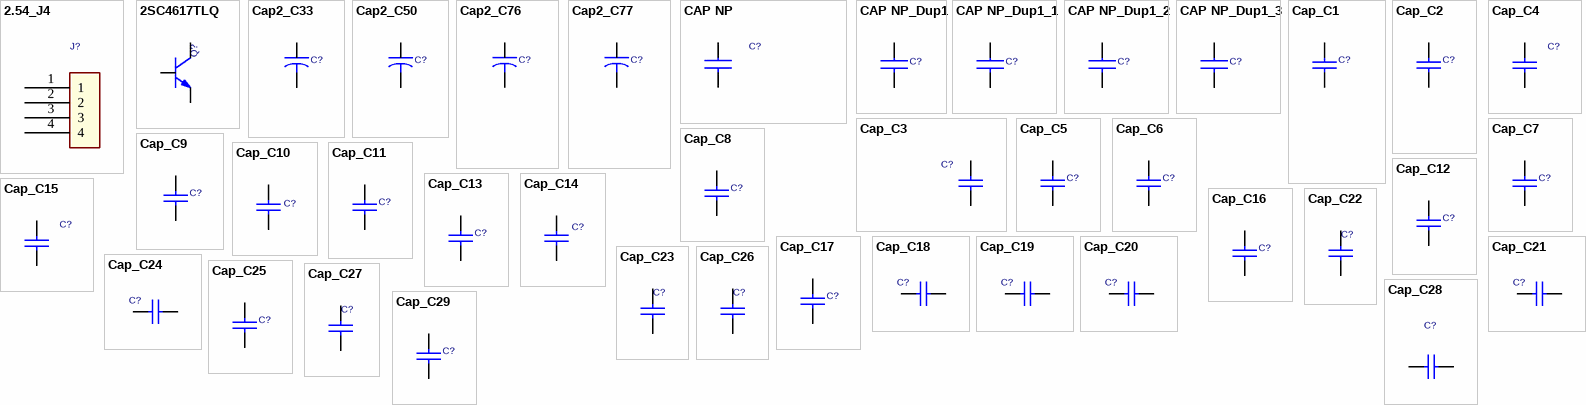
[diagram p0: symbols 2.54_J4 to Cap_C29]
# Altium schematic symbol library MISC86294-22.SCHLIB: 224 symbols
Pins are listed as number, name and electrical type; pins without a type are passive.


## 2.54_J4
designator J?
footprint HDR1X4
pins: 1, 2, 3, 4

## 2SC4617TLQ
designator Q?
simulation model 2SC4617TLQ
footprint EMT3
pins: 1 E, 2 B, 3 C

## Cap2_C33
designator C?
footprint CAP-TH_BD5_0-P2_00-D0_8-FD
pins: 1, 2

## Cap2_C50
designator C?
footprint C0805
pins: 1, 2

## Cap2_C76
designator C?
footprint RB5*7
pins: 1, 2

## Cap2_C77
designator C?
footprint RB5*7
pins: 1, 2

## CAP NP
designator C?
footprint 0603
pins: 1, 2

## CAP NP_Dup1
designator C?
footprint C0603
pins: 1, 2

## CAP NP_Dup1_1
designator C?
footprint C0603
pins: 1, 2

## CAP NP_Dup1_2
designator C?
footprint C0603
pins: 1, 2

## CAP NP_Dup1_3
designator C?
footprint C0805
pins: 1, 2

## Cap_C1
designator C?
footprint C0805
pins: 1, 2

## Cap_C2
designator C?
footprint C0805
pins: 1, 2

## Cap_C3
designator C?
footprint C0805
pins: 1, 2

## Cap_C4
designator C?
footprint C0805
pins: 1, 2

## Cap_C5
designator C?
footprint 0603
footprint C0603
pins: 1, 2

## Cap_C6
designator C?
footprint 0603
footprint C0603
pins: 1, 2

## Cap_C7
designator C?
footprint 0603
footprint C0603
pins: 1, 2

## Cap_C8
designator C?
footprint 0603
footprint C0603
pins: 1, 2

## Cap_C9
designator C?
footprint 0603
footprint C0603
pins: 1, 2

## Cap_C10
designator C?
footprint 0603
footprint C0603
pins: 1, 2

## Cap_C11
designator C?
footprint 0603
footprint C0603
pins: 1, 2

## Cap_C12
designator C?
footprint 0603
footprint C0603
pins: 1, 2

## Cap_C13
designator C?
footprint 0603
footprint C0603
pins: 1, 2

## Cap_C14
designator C?
footprint 0603
footprint C0603
pins: 1, 2

## Cap_C15
designator C?
footprint C0805
pins: 1, 2

## Cap_C16
designator C?
footprint 0603
footprint C0603
pins: 1, 2

## Cap_C17
designator C?
footprint 0603
footprint C0603
pins: 1, 2

## Cap_C18
designator C?
footprint 0603
pins: 1, 2

## Cap_C19
designator C?
footprint 0603
pins: 1, 2

## Cap_C20
designator C?
footprint 0603
pins: 1, 2

## Cap_C21
designator C?
footprint 0603
pins: 1, 2

## Cap_C22
designator C?
footprint 0603
pins: 1, 2

## Cap_C23
designator C?
footprint 0603
pins: 1, 2

## Cap_C24
designator C?
footprint 0603
pins: 1, 2

## Cap_C25
designator C?
footprint CAP-TH_BD8_0-P3_50-D1_0-FD
pins: 1, 2

## Cap_C26
designator C?
footprint 0603
pins: 1, 2

## Cap_C27
designator C?
footprint 0603
pins: 1, 2

## Cap_C28
designator C?
footprint 0603
footprint C0603
pins: 1, 2

## Cap_C29
designator C?
footprint 0603
footprint C0603
pins: 1, 2

## Cap_C30
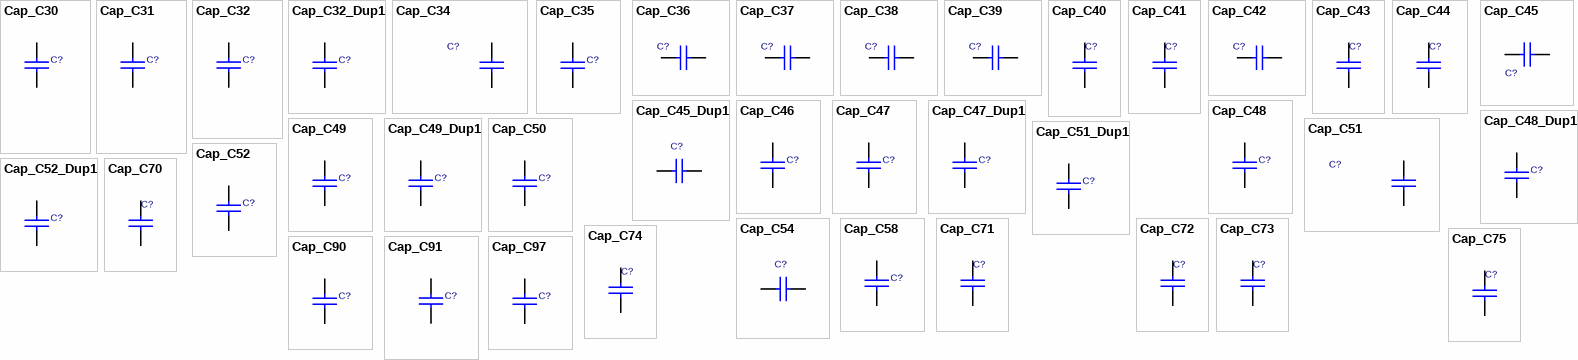
[diagram p1: symbols Cap_C30 to Cap_C97]
## Cap_C30
designator C?
footprint C0805
pins: 1, 2

## Cap_C31
designator C?
footprint 0603
footprint C0603
pins: 1, 2

## Cap_C32
designator C?
footprint C0805
pins: 1, 2

## Cap_C32_Dup1
designator C?
footprint C0603
pins: 1, 2

## Cap_C34
designator C?
footprint C0805
pins: 1, 2

## Cap_C35
designator C?
footprint 0603
footprint C0603
pins: 1, 2

## Cap_C36
designator C?
footprint 0603
pins: 1, 2

## Cap_C37
designator C?
footprint 0603
pins: 1, 2

## Cap_C38
designator C?
footprint 0603
pins: 1, 2

## Cap_C39
designator C?
footprint 0603
pins: 1, 2

## Cap_C40
designator C?
footprint 0603
pins: 1, 2

## Cap_C41
designator C?
footprint 0603
pins: 1, 2

## Cap_C42
designator C?
footprint 0603
pins: 1, 2

## Cap_C43
designator C?
footprint 0603
pins: 1, 2

## Cap_C44
designator C?
footprint 0603
pins: 1, 2

## Cap_C45
designator C?
footprint 0603
footprint C0603
pins: 1, 2

## Cap_C45_Dup1
designator C?
footprint C0603
pins: 1, 2

## Cap_C46
designator C?
footprint 0603
footprint C0603
pins: 1, 2

## Cap_C47
designator C?
footprint C0805
pins: 1, 2

## Cap_C47_Dup1
designator C?
footprint C0603
pins: 1, 2

## Cap_C48
designator C?
footprint 0603
footprint C0603
pins: 1, 2

## Cap_C48_Dup1
designator C?
footprint C0603
pins: 1, 2

## Cap_C49
designator C?
footprint C0805
pins: 1, 2

## Cap_C49_Dup1
designator C?
footprint C0603
pins: 1, 2

## Cap_C50
designator C?
footprint C0603
pins: 1, 2

## Cap_C51
designator C?
footprint C0805
pins: 1, 2

## Cap_C51_Dup1
designator C?
footprint C0603
pins: 1, 2

## Cap_C52
designator C?
footprint 0603
footprint C0603
pins: 1, 2

## Cap_C52_Dup1
designator C?
footprint C0603
pins: 1, 2

## Cap_C54
designator C?
footprint C0603
pins: 1, 2

## Cap_C58
designator C?
footprint C0603
pins: 1, 2

## Cap_C70
designator C?
footprint C0603
pins: 1, 2

## Cap_C71
designator C?
footprint C0603
pins: 1, 2

## Cap_C72
designator C?
footprint C0603
pins: 1, 2

## Cap_C73
designator C?
footprint C0603
pins: 1, 2

## Cap_C74
designator C?
footprint C0603
pins: 1, 2

## Cap_C75
designator C?
footprint C0603
pins: 1, 2

## Cap_C90
designator C?
footprint C0603
pins: 1, 2

## Cap_C91
designator C?
footprint RB8*11_5
pins: 1, 2

## Cap_C97
designator C?
footprint C0603
pins: 1, 2

## Cap_C98
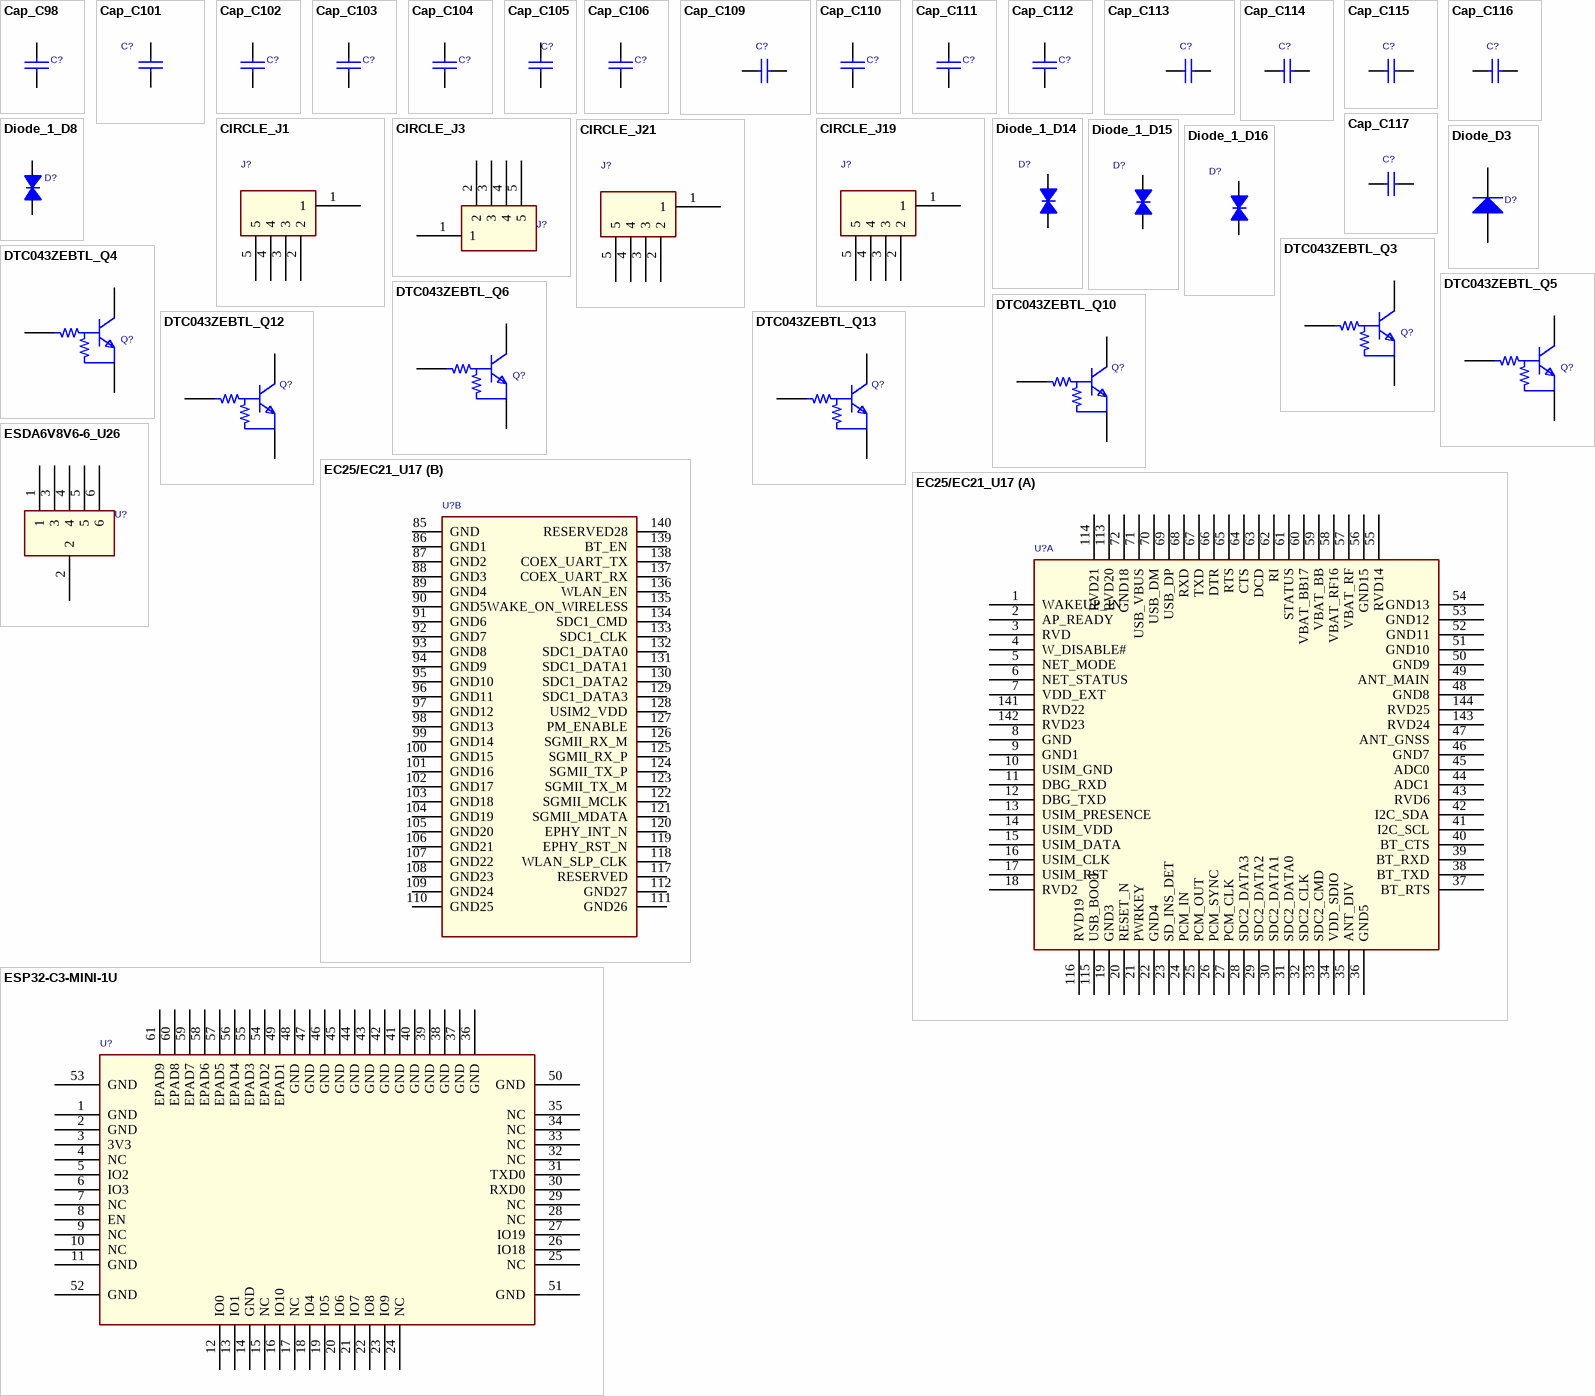
[diagram p2: symbols Cap_C98 to ESP32-C3-MINI-1U]
## Cap_C98
designator C?
footprint C0603
pins: 1, 2

## Cap_C101
designator C?
footprint C0603
pins: 1, 2

## Cap_C102
designator C?
footprint C0603
pins: 1, 2

## Cap_C103
designator C?
footprint C0603
pins: 1, 2

## Cap_C104
designator C?
footprint RB8*11_5
pins: 1, 2

## Cap_C105
designator C?
footprint C0603
pins: 1, 2

## Cap_C106
designator C?
footprint C0603
pins: 1, 2

## Cap_C109
designator C?
footprint C0603
pins: 1, 2

## Cap_C110
designator C?
footprint C0603
pins: 1, 2

## Cap_C111
designator C?
footprint C0603
pins: 1, 2

## Cap_C112
designator C?
footprint C0603
pins: 1, 2

## Cap_C113
designator C?
footprint C0603
pins: 1, 2

## Cap_C114
designator C?
footprint C0603
pins: 1, 2

## Cap_C115
designator C?
footprint C0603
pins: 1, 2

## Cap_C116
designator C?
footprint C0603
pins: 1, 2

## Cap_C117
designator C?
footprint C0603
pins: 1, 2

## CIRCLE_J1
designator J?
footprint MMCX-TH_ZC11_801KK
pins: 1, 2, 3, 4, 5

## CIRCLE_J3
designator J?
footprint MMCX-TH_ZC11_801KK
pins: 1, 2, 3, 4, 5

## CIRCLE_J19
designator J?
footprint MMCX-KE
pins: 1, 2, 3, 4, 5

## CIRCLE_J21
designator J?
footprint MMCX-KE
pins: 1, 2, 3, 4, 5

## Diode_1_D8
designator D?
footprint SMA
pins: 1 A, 2 K

## Diode_1_D14
designator D?
footprint SMA
pins: 1 A, 2 K

## Diode_1_D15
designator D?
footprint SMA
pins: 1 A, 2 K

## Diode_1_D16
designator D?
footprint SMA
pins: 1 A, 2 K

## Diode_D3
designator D?
footprint SMC_L6_9-W5_9-LS7_9-RD
pins: 1 A, 2 K

## DTC043ZEBTL_Q3
designator Q?
footprint SOT-416_L1_6-W0_8-P1_00-LS1_6-BR
pins: 1 B, 2 E, 3 C

## DTC043ZEBTL_Q4
designator Q?
footprint SOT-416_L1_6-W0_8-P1_00-LS1_6-BR
pins: 1 B, 2 E, 3 C

## DTC043ZEBTL_Q5
designator Q?
footprint SOT-416_L1_6-W0_8-P1_00-LS1_6-BR
pins: 1 B, 2 E, 3 C

## DTC043ZEBTL_Q6
designator Q?
footprint SOT-416_L1_6-W0_8-P1_00-LS1_6-BR
pins: 1 B, 2 E, 3 C

## DTC043ZEBTL_Q10
designator Q?
footprint SOT-416_L1_6-W0_8-P1_00-LS1_6-BR
pins: 1 B, 2 E, 3 C

## DTC043ZEBTL_Q12
designator Q?
footprint SOT-416_L1_6-W0_8-P1_00-LS1_6-BR
pins: 1 B, 2 E, 3 C

## DTC043ZEBTL_Q13
designator Q?
footprint SOT-416_L1_6-W0_8-P1_00-LS1_6-BR
pins: 1 B, 2 E, 3 C

## EC25/EC21_U17
designator U?
footprint EC20
part A pins: 1 WAKEUP_IN, 2 AP_READY, 3 RVD, 4 W_DISABLE#, 5 NET_MODE, 6 NET_STATUS, 7 VDD_EXT, 8 GND, 9 GND1, 10 USIM_GND, 11 DBG_RXD, 12 DBG_TXD, 13 USIM_PRESENCE, 14 USIM_VDD, 15 USIM_DATA, 16 USIM_CLK, 17 USIM_RST, 18 RVD2, 19 GND3, 20 RESET_N, 21 PWRKEY, 22 GND4, 23 SD_INS_DET, 24 PCM_IN, 25 PCM_OUT, 26 PCM_SYNC, 27 PCM_CLK, 28 SDC2_DATA3, 29 SDC2_DATA2, 30 SDC2_DATA1, 31 SDC2_DATA0, 32 SDC2_CLK, 33 SDC2_CMD, 34 VDD_SDIO, 35 ANT_DIV, 36 GND5, 37 BT_RTS, 38 BT_TXD, 39 BT_RXD, 40 BT_CTS, 41 I2C_SCL, 42 I2C_SDA, 43 RVD6, 44 ADC1, 45 ADC0, 46 GND7, 47 ANT_GNSS, 48 GND8, 49 ANT_MAIN, 50 GND9, 51 GND10, 52 GND11, 53 GND12, 54 GND13, 55 RVD14, 56 GND15, 57 VBAT_RF, 58 VBAT_RF16, 59 VBAT_BB, 60 VBAT_BB17, 61 STATUS, 62 RI, 63 DCD, 64 CTS, 65 RTS, 66 DTR, 67 TXD, 68 RXD, 69 USB_DP, 70 USB_DM, 71 USB_VBUS, 72 GND18, 113 RVD20, 114 RVD21, 115 USB_BOOT, 116 RVD19, 141 RVD22, 142 RVD23, 143 RVD24, 144 RVD25
part B pins: 85 GND, 86 GND1, 87 GND2, 88 GND3, 89 GND4, 90 GND5, 91 GND6, 92 GND7, 93 GND8, 94 GND9, 95 GND10, 96 GND11, 97 GND12, 98 GND13, 99 GND14, 100 GND15, 101 GND16, 102 GND17, 103 GND18, 104 GND19, 105 GND20, 106 GND21, 107 GND22, 108 GND23, 109 GND24, 110 GND25, 111 GND26, 112 GND27, 117 RESERVED, 118 WLAN_SLP_CLK, 119 EPHY_RST_N, 120 EPHY_INT_N, 121 SGMII_MDATA, 122 SGMII_MCLK, 123 SGMII_TX_M, 124 SGMII_TX_P, 125 SGMII_RX_P, 126 SGMII_RX_M, 127 PM_ENABLE, 128 USIM2_VDD, 129 SDC1_DATA3, 130 SDC1_DATA2, 131 SDC1_DATA1, 132 SDC1_DATA0, 133 SDC1_CLK, 134 SDC1_CMD, 135 WAKE_ON_WIRELESS, 136 WLAN_EN, 137 COEX_UART_RX, 138 COEX_UART_TX, 139 BT_EN, 140 RESERVED28

## ESDA6V8V6-6_U26
designator U?
footprint SOT-563
pins: 1, 2, 3, 4, 5, 6

## ESP32-C3-MINI-1U
designator U?
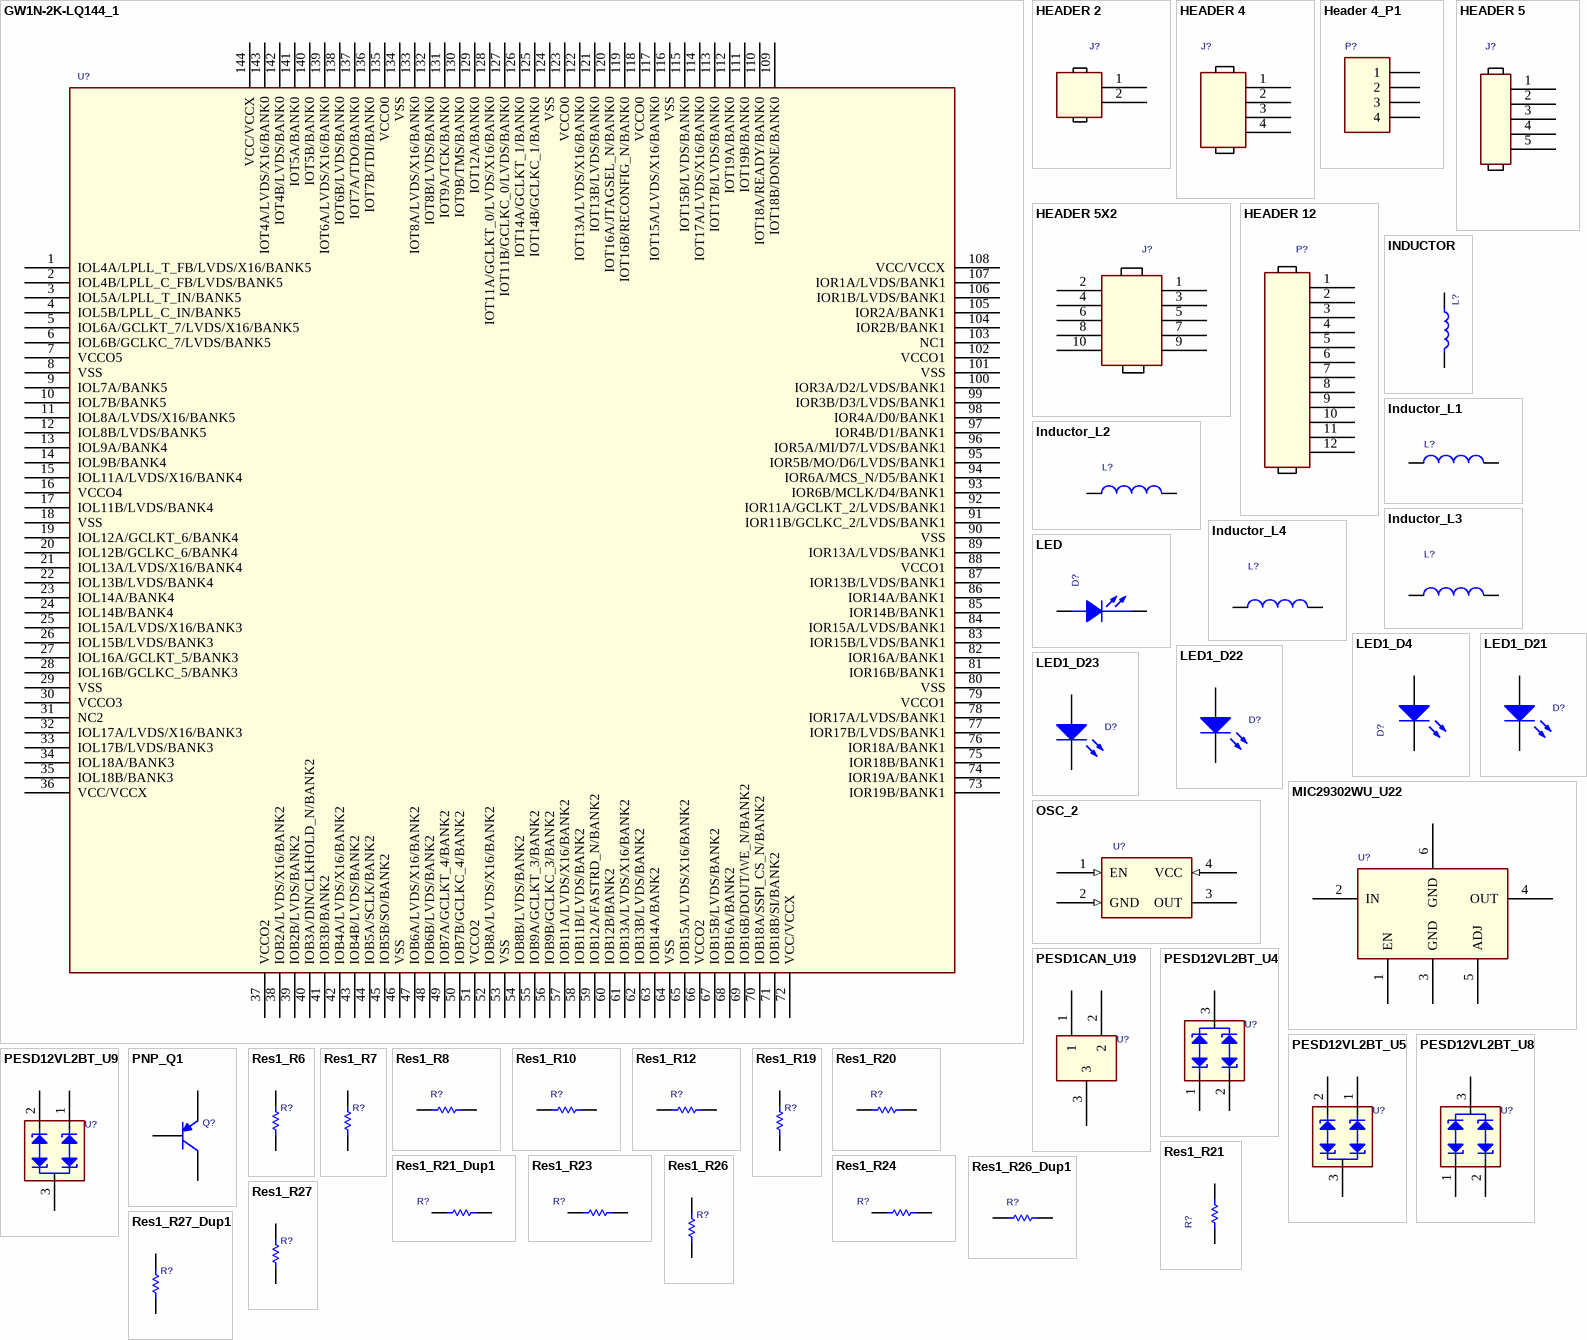
[diagram p3: symbols GW1N-2K-LQ144_1 to Res1_R27_Dup1]
pins: 1 GND, 2 GND, 3 3V3, 4 NC, 5 IO2, 6 IO3, 7 NC, 8 EN, 9 NC, 10 NC, 11 GND, 12 IO0, 13 IO1, 14 GND, 15 NC, 16 IO10, 17 NC, 18 IO4, 19 IO5, 20 IO6, 21 IO7, 22 IO8, 23 IO9, 24 NC, 25 NC, 26 IO18, 27 IO19, 28 NC, 29 NC, 30 RXD0, 31 TXD0, 32 NC, 33 NC, 34 NC, 35 NC, 36 GND, 37 GND, 38 GND, 39 GND, 40 GND, 41 GND, 42 GND, 43 GND, 44 GND, 45 GND, 46 GND, 47 GND, 48 GND, 49 EPAD1, 50 GND, 51 GND, 52 GND, 53 GND, 54 EPAD2, 55 EPAD3, 56 EPAD4, 57 EPAD5, 58 EPAD6, 59 EPAD7, 60 EPAD8, 61 EPAD9


## GW1N-2K-LQ144_1
designator U?
footprint LQ144_1
pins: 1 IOL4A/LPLL_T_FB/LVDS/X16/BANK5, 2 IOL4B/LPLL_C_FB/LVDS/BANK5, 3 IOL5A/LPLL_T_IN/BANK5, 4 IOL5B/LPLL_C_IN/BANK5, 5 IOL6A/GCLKT_7/LVDS/X16/BANK5, 6 IOL6B/GCLKC_7/LVDS/BANK5, 7 VCCO5 (power), 8 VSS (power), 9 IOL7A/BANK5, 10 IOL7B/BANK5, 11 IOL8A/LVDS/X16/BANK5, 12 IOL8B/LVDS/BANK5, 13 IOL9A/BANK4, 14 IOL9B/BANK4, 15 IOL11A/LVDS/X16/BANK4, 16 VCCO4 (power), 17 IOL11B/LVDS/BANK4, 18 VSS (power), 19 IOL12A/GCLKT_6/BANK4, 20 IOL12B/GCLKC_6/BANK4, 21 IOL13A/LVDS/X16/BANK4, 22 IOL13B/LVDS/BANK4, 23 IOL14A/BANK4, 24 IOL14B/BANK4, 25 IOL15A/LVDS/X16/BANK3, 26 IOL15B/LVDS/BANK3, 27 IOL16A/GCLKT_5/BANK3, 28 IOL16B/GCLKC_5/BANK3, 29 VSS (power), 30 VCCO3 (power), 31 NC2, 32 IOL17A/LVDS/X16/BANK3, 33 IOL17B/LVDS/BANK3, 34 IOL18A/BANK3, 35 IOL18B/BANK3, 36 VCC/VCCX (power), 37 VCCO2 (power), 38 IOB2A/LVDS/X16/BANK2, 39 IOB2B/LVDS/BANK2, 40 IOB3A/DIN/CLKHOLD_N/BANK2, 41 IOB3B/BANK2, 42 IOB4A/LVDS/X16/BANK2, 43 IOB4B/LVDS/BANK2, 44 IOB5A/SCLK/BANK2, 45 IOB5B/SO/BANK2, 46 VSS (power), 47 IOB6A/LVDS/X16/BANK2, 48 IOB6B/LVDS/BANK2, 49 IOB7A/GCLKT_4/BANK2, 50 IOB7B/GCLKC_4/BANK2, 51 VCCO2 (power), 52 IOB8A/LVDS/X16/BANK2, 53 VSS (power), 54 IOB8B/LVDS/BANK2, 55 IOB9A/GCLKT_3/BANK2, 56 IOB9B/GCLKC_3/BANK2, 57 IOB11A/LVDS/X16/BANK2, 58 IOB11B/LVDS/BANK2, 59 IOB12A/FASTRD_N/BANK2, 60 IOB12B/BANK2, 61 IOB13A/LVDS/X16/BANK2, 62 IOB13B/LVDS/BANK2, 63 IOB14A/BANK2, 64 VSS (power), 65 IOB15A/LVDS/X16/BANK2, 66 VCCO2 (power), 67 IOB15B/LVDS/BANK2, 68 IOB16A/BANK2, 69 IOB16B/DOUT/WE_N/BANK2, 70 IOB18A/SSPI_CS_N/BANK2, 71 IOB18B/SI/BANK2, 72 VCC/VCCX (power), 73 IOR19B/BANK1, 74 IOR19A/BANK1, 75 IOR18B/BANK1, 76 IOR18A/BANK1, 77 IOR17B/LVDS/BANK1, 78 IOR17A/LVDS/BANK1, 79 VCCO1 (power), 80 VSS (power), 81 IOR16B/BANK1, 82 IOR16A/BANK1, 83 IOR15B/LVDS/BANK1, 84 IOR15A/LVDS/BANK1, 85 IOR14B/BANK1, 86 IOR14A/BANK1, 87 IOR13B/LVDS/BANK1, 88 VCCO1 (power), 89 IOR13A/LVDS/BANK1, 90 VSS (power), 91 IOR11B/GCLKC_2/LVDS/BANK1, 92 IOR11A/GCLKT_2/LVDS/BANK1, 93 IOR6B/MCLK/D4/BANK1, 94 IOR6A/MCS_N/D5/BANK1, 95 IOR5B/MO/D6/LVDS/BANK1, 96 IOR5A/MI/D7/LVDS/BANK1, 97 IOR4B/D1/BANK1, 98 IOR4A/D0/BANK1, 99 IOR3B/D3/LVDS/BANK1, 100 IOR3A/D2/LVDS/BANK1, 101 VSS (power), 102 VCCO1 (power), 103 NC1, 104 IOR2B/BANK1, 105 IOR2A/BANK1, 106 IOR1B/LVDS/BANK1, 107 IOR1A/LVDS/BANK1, 108 VCC/VCCX (power), 109 IOT18B/DONE/BANK0, 110 IOT18A/READY/BANK0, 111 IOT19B/BANK0, 112 IOT19A/BANK0, 113 IOT17B/LVDS/BANK0, 114 IOT17A/LVDS/X16/BANK0, 115 IOT15B/LVDS/BANK0, 116 VSS (power), 117 IOT15A/LVDS/X16/BANK0, 118 VCCO0 (power), 119 IOT16B/RECONFIG_N/BANK0, 120 IOT16A/JTAGSEL_N/BANK0, 121 IOT13B/LVDS/BANK0, 122 IOT13A/LVDS/X16/BANK0, 123 VCCO0 (power), 124 VSS (power), 125 IOT14B/GCLKC_1/BANK0, 126 IOT14A/GCLKT_1/BANK0, 127 IOT11B/GCLKC_0/LVDS/BANK0, 128 IOT11A/GCLKT_0/LVDS/X16/BANK0, 129 IOT12A/BANK0, 130 IOT9B/TMS/BANK0, 131 IOT9A/TCK/BANK0, 132 IOT8B/LVDS/BANK0, 133 IOT8A/LVDS/X16/BANK0, 134 VSS (power), 135 VCCO0 (power), 136 IOT7B/TDI/BANK0, 137 IOT7A/TDO/BANK0, 138 IOT6B/LVDS/BANK0, 139 IOT6A/LVDS/X16/BANK0, 140 IOT5B/BANK0, 141 IOT5A/BANK0, 142 IOT4B/LVDS/BANK0, 143 IOT4A/LVDS/X16/BANK0, 144 VCC/VCCX (power)

## HEADER 2
designator J?
pins: 1, 2

## HEADER 4
designator J?
pins: 1, 2, 3, 4

## Header 4_P1
designator P?
footprint HDR1X4
pins: 1, 2, 3, 4

## HEADER 5
designator J?
footprint 2.54mm_paizhen_5pin
pins: 1, 2, 3, 4, 5

## HEADER 5X2
designator J?
pins: 1, 2, 3, 4, 5, 6, 7, 8, 9, 10

## HEADER 12
designator P?
pins: 1, 2, 3, 4, 5, 6, 7, 8, 9, 10, 11, 12

## INDUCTOR
designator L?
footprint 0805
pins: 1, 2

## Inductor_L1
designator L?
footprint 1210
pins: 1, 2

## Inductor_L2
designator L?
footprint 0603
footprint R0603
pins: 1, 2

## Inductor_L3
designator L?
footprint IND-SMD_L4_0-W4_0
pins: 1, 2

## Inductor_L4
designator L?
footprint IND-SMD_L4_0-W4_0
pins: 1, 2

## LED
designator D?
footprint LED0603
pins: 1 CATHODE, 2 ANODE

## LED1_D4
designator D?
footprint LED_0805
footprint LED0603
pins: 1 A, 2 K

## LED1_D21
designator D?
footprint LED0805
pins: 1 A, 2 K

## LED1_D22
designator D?
footprint LED0805
pins: 1 A, 2 K

## LED1_D23
designator D?
footprint LED0805
pins: 1 A, 2 K

## MIC29302WU_U22
designator U?
footprint TO-263-5
pins: 1 EN, 2 IN, 3 GND, 4 OUT, 5 ADJ, 6 GND

## OSC_2
designator U?
100Mhz Oscillator half can
footprint SMD3225
pins: 1 EN (in), 2 GND (in), 3 OUT, 4 VCC (in)

## PESD1CAN_U19
designator U?
footprint SOT-23-3
pins: 1, 2, 3

## PESD12VL2BT_U4
designator U?
footprint SOT-23
pins: 1, 2, 3

## PESD12VL2BT_U5
designator U?
footprint SOT-23
pins: 1, 2, 3

## PESD12VL2BT_U8
designator U?
footprint SOT-23
pins: 1, 2, 3

## PESD12VL2BT_U9
designator U?
footprint SOT-23
pins: 1, 2, 3

## PNP_Q1
designator Q?
footprint SOT-23-SS8550
pins: 1 B, 2 E, 3 C

## Res1_R6
designator R?
footprint 0603
pins: 1, 2

## Res1_R7
designator R?
footprint 0603
pins: 1, 2

## Res1_R8
designator R?
footprint 0603
pins: 1, 2

## Res1_R10
designator R?
footprint 0603
pins: 1, 2

## Res1_R12
designator R?
footprint 0603
pins: 1, 2

## Res1_R19
designator R?
footprint 0603
footprint R0603
pins: 1, 2

## Res1_R20
designator R?
footprint 0603
footprint R0603
pins: 1, 2

## Res1_R21
designator R?
footprint 0603
pins: 1, 2

## Res1_R21_Dup1
designator R?
footprint R0603
pins: 1, 2

## Res1_R23
designator R?
footprint R0603
pins: 1, 2

## Res1_R24
designator R?
footprint R0603
pins: 1, 2

## Res1_R26
designator R?
footprint 0603
footprint R0603
pins: 1, 2

## Res1_R26_Dup1
designator R?
footprint R0603
pins: 1, 2

## Res1_R27
designator R?
footprint 0603
footprint R0603
pins: 1, 2

## Res1_R27_Dup1
designator R?
footprint R0603
pins: 1, 2

## Res1_R28
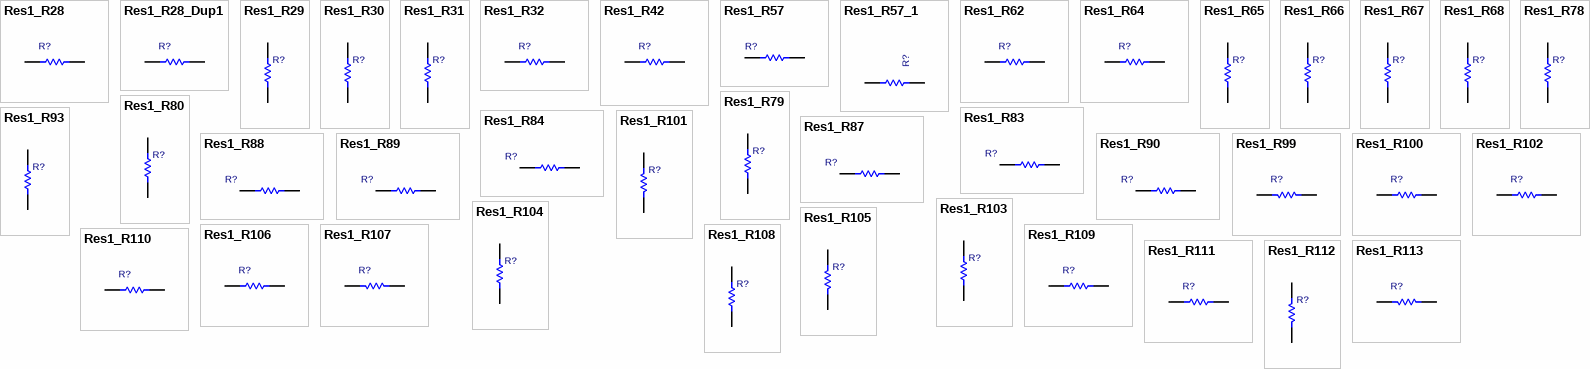
[diagram p4: symbols Res1_R28 to Res1_R113]
## Res1_R28
designator R?
footprint 0603
footprint R0603
pins: 1, 2

## Res1_R28_Dup1
designator R?
footprint R0603
pins: 1, 2

## Res1_R29
designator R?
footprint 0603
footprint R0603
pins: 1, 2

## Res1_R30
designator R?
footprint R0603
pins: 1, 2

## Res1_R31
designator R?
footprint R0603
pins: 1, 2

## Res1_R32
designator R?
footprint R0603
pins: 1, 2

## Res1_R42
designator R?
footprint R0603
pins: 1, 2

## Res1_R57
designator R?
footprint R0603
pins: 1, 2

## Res1_R57_1
designator R?
footprint R0603
pins: 1, 2

## Res1_R62
designator R?
footprint R0603
pins: 1, 2

## Res1_R64
designator R?
footprint R0603
pins: 1, 2

## Res1_R65
designator R?
footprint R0603
pins: 1, 2

## Res1_R66
designator R?
footprint R0603
pins: 1, 2

## Res1_R67
designator R?
footprint R0603
pins: 1, 2

## Res1_R68
designator R?
footprint R0603
pins: 1, 2

## Res1_R78
designator R?
footprint R0603
pins: 1, 2

## Res1_R79
designator R?
footprint R0603
pins: 1, 2

## Res1_R80
designator R?
footprint R0603
pins: 1, 2

## Res1_R83
designator R?
footprint R0603
pins: 1, 2

## Res1_R84
designator R?
footprint R0603
pins: 1, 2

## Res1_R87
designator R?
footprint R0603
pins: 1, 2

## Res1_R88
designator R?
footprint R0603
pins: 1, 2

## Res1_R89
designator R?
footprint R0603
pins: 1, 2

## Res1_R90
designator R?
footprint R0603
pins: 1, 2

## Res1_R93
designator R?
footprint R0603
pins: 1, 2

## Res1_R99
designator R?
footprint R0603
pins: 1, 2

## Res1_R100
designator R?
footprint R0603
pins: 1, 2

## Res1_R101
designator R?
footprint R0603
pins: 1, 2

## Res1_R102
designator R?
footprint R0603
pins: 1, 2

## Res1_R103
designator R?
footprint R0603
pins: 1, 2

## Res1_R104
designator R?
footprint R0603
pins: 1, 2

## Res1_R105
designator R?
footprint R0603
pins: 1, 2

## Res1_R106
designator R?
footprint R0603
pins: 1, 2

## Res1_R107
designator R?
footprint R0603
pins: 1, 2

## Res1_R108
designator R?
footprint R0603
pins: 1, 2

## Res1_R109
designator R?
footprint R0603
pins: 1, 2

## Res1_R110
designator R?
footprint R0603
pins: 1, 2

## Res1_R111
designator R?
footprint R0603
pins: 1, 2

## Res1_R112
designator R?
footprint R0603
pins: 1, 2

## Res1_R113
designator R?
footprint R0603
pins: 1, 2

## Res1_R114
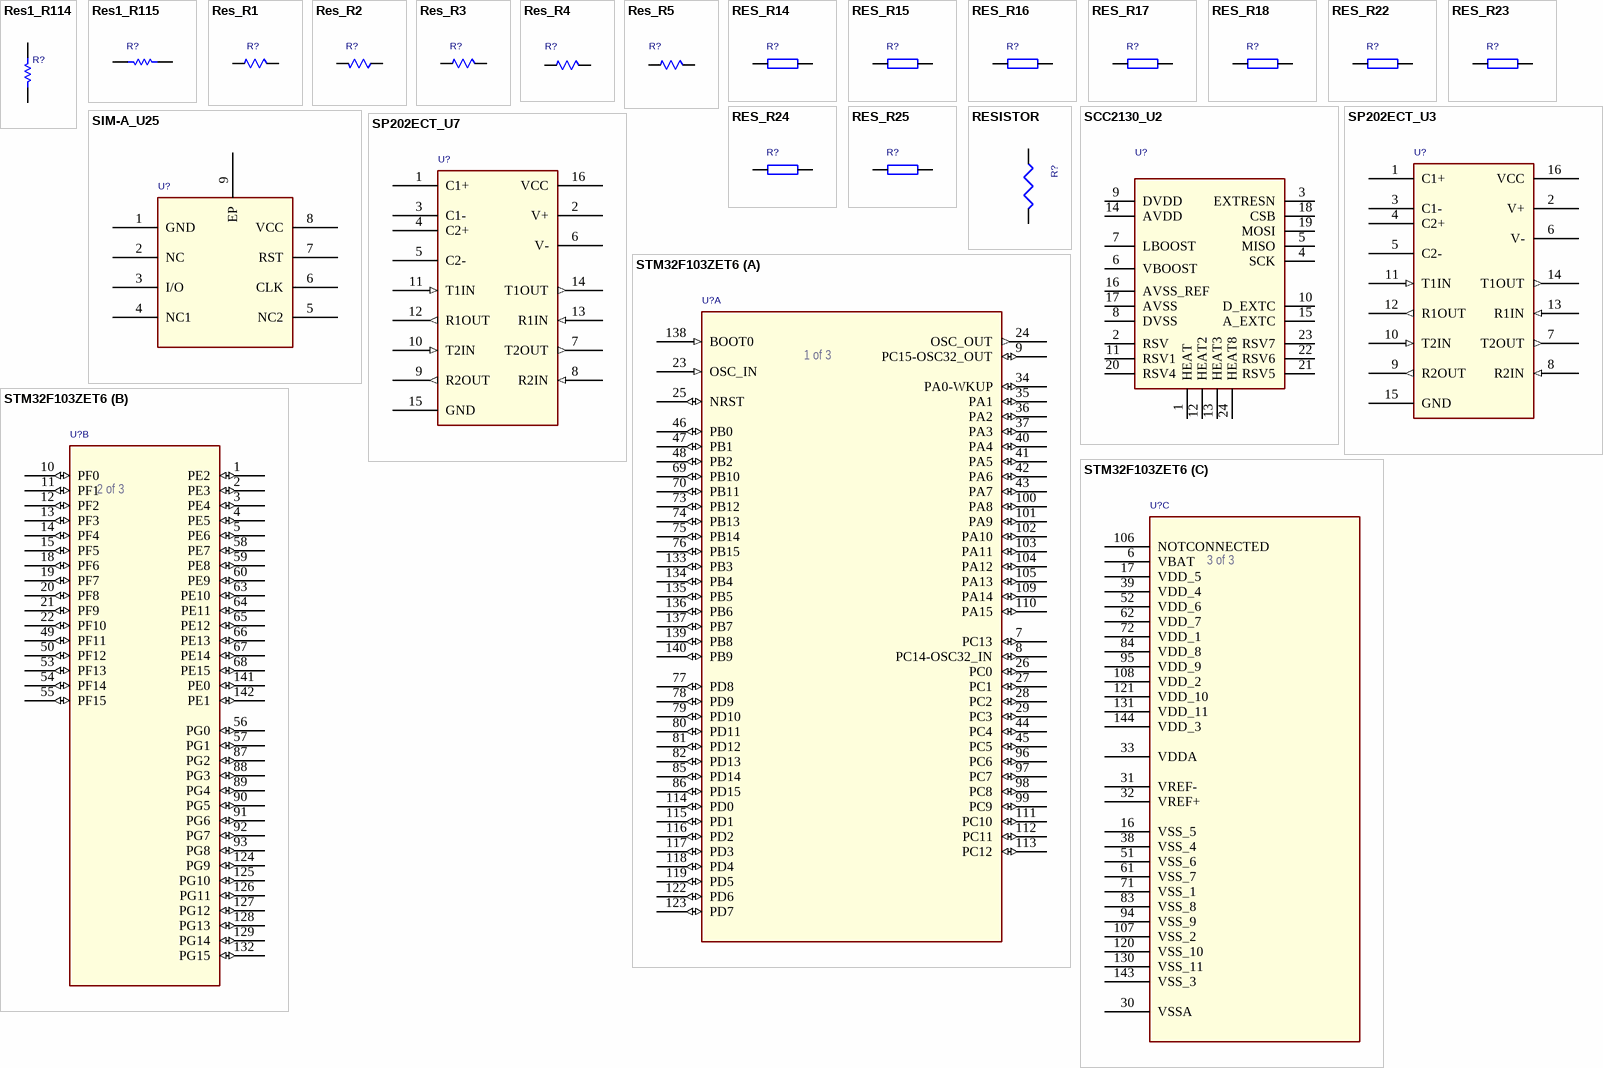
[diagram p5: symbols Res1_R114 to STM32F103ZET6]
## Res1_R114
designator R?
footprint R0603
pins: 1, 2

## Res1_R115
designator R?
footprint R0603
pins: 1, 2

## Res_R1
designator R?
footprint 0603
pins: 1, 2

## Res_R2
designator R?
footprint 0603
pins: 1, 2

## Res_R3
designator R?
footprint 0603
pins: 1, 2

## Res_R4
designator R?
footprint 0603
pins: 1, 2

## Res_R5
designator R?
footprint 0603
pins: 1, 2

## RES_R14
designator R?
footprint 0603
pins: 1, 2

## RES_R15
designator R?
footprint 1210
footprint R1210
pins: 1, 2

## RES_R16
designator R?
footprint 0603
pins: 1, 2

## RES_R17
designator R?
footprint 0603
pins: 1, 2

## RES_R18
designator R?
footprint 0603
pins: 1, 2

## RES_R22
designator R?
footprint 0603
pins: 1, 2

## RES_R23
designator R?
footprint 0603
pins: 1, 2

## RES_R24
designator R?
footprint 0603
pins: 1, 2

## RES_R25
designator R?
footprint 0603
pins: 1, 2

## RESISTOR
designator R?
footprint 0603
pins: 1, 2

## SCC2130_U2
designator U?
footprint SCC2130D
pins: 1 HEAT, 2 RSV, 3 EXTRESN, 4 SCK, 5 MISO, 6 VBOOST, 7 LBOOST, 8 DVSS, 9 DVDD, 10 D_EXTC, 11 RSV1, 12 HEAT2, 13 HEAT3, 14 AVDD, 15 A_EXTC, 16 AVSS_REF, 17 AVSS, 18 CSB, 19 MOSI, 20 RSV4, 21 RSV5, 22 RSV6, 23 RSV7, 24 HEAT8

## SIM-A_U25
designator U?
footprint DFN2*2-8
pins: 1 GND, 2 NC, 3 I/O, 4 NC1, 5 NC2, 6 CLK, 7 RST, 8 VCC, 9 EP

## SP202ECT_U3
designator U?
footprint SOP16-6_6
pins: 1 C1+, 2 V+, 3 C1-, 4 C2+, 5 C2-, 6 V-, 7 T2OUT (out), 8 R2IN (in), 9 R2OUT (out), 10 T2IN (in), 11 T1IN (in), 12 R1OUT (out), 13 R1IN (in), 14 T1OUT (out), 15 GND, 16 VCC

## SP202ECT_U7
designator U?
footprint SOP16-6_6
pins: 1 C1+, 2 V+, 3 C1-, 4 C2+, 5 C2-, 6 V-, 7 T2OUT (out), 8 R2IN (in), 9 R2OUT (out), 10 T2IN (in), 11 T1IN (in), 12 R1OUT (out), 13 R1IN (in), 14 T1OUT (out), 15 GND, 16 VCC

## STM32F103ZET6
designator U?
footprint LQFP144-20x20mm
part A pins: 7 PC13 (io), 8 PC14-OSC32_IN (io), 9 PC15-OSC32_OUT (io), 23 OSC_IN (in), 24 OSC_OUT (out), 25 NRST (io), 26 PC0 (io), 27 PC1 (io), 28 PC2 (io), 29 PC3 (io), 34 PA0-WKUP (io), 35 PA1 (io), 36 PA2 (io), 37 PA3 (io), 40 PA4 (io), 41 PA5 (io), 42 PA6 (io), 43 PA7 (io), 44 PC4 (io), 45 PC5 (io), 46 PB0 (io), 47 PB1 (io), 48 PB2 (io), 69 PB10 (io), 70 PB11 (io), 73 PB12 (io), 74 PB13 (io), 75 PB14 (io), 76 PB15 (io), 77 PD8 (io), 78 PD9 (io), 79 PD10 (io), 80 PD11 (io), 81 PD12 (io), 82 PD13 (io), 85 PD14 (io), 86 PD15 (io), 96 PC6 (io), 97 PC7 (io), 98 PC8 (io), 99 PC9 (io), 100 PA8 (io), 101 PA9 (io), 102 PA10 (io), 103 PA11 (io), 104 PA12 (io), 105 PA13 (io), 109 PA14 (io), 110 PA15 (io), 111 PC10 (io), 112 PC11 (io), 113 PC12 (io), 114 PD0 (io), 115 PD1 (io), 116 PD2 (io), 117 PD3 (io), 118 PD4 (io), 119 PD5 (io), 122 PD6 (io), 123 PD7 (io), 133 PB3 (io), 134 PB4 (io), 135 PB5 (io), 136 PB6 (io), 137 PB7 (io), 138 BOOT0 (in), 139 PB8 (io), 140 PB9 (io)
part B pins: 1 PE2 (io), 2 PE3 (io), 3 PE4 (io), 4 PE5 (io), 5 PE6 (io), 10 PF0 (io), 11 PF1 (io), 12 PF2 (io), 13 PF3 (io), 14 PF4 (io), 15 PF5 (io), 18 PF6 (io), 19 PF7 (io), 20 PF8 (io), 21 PF9 (io), 22 PF10 (io), 49 PF11 (io), 50 PF12 (io), 53 PF13 (io), 54 PF14 (io), 55 PF15 (io), 56 PG0 (io), 57 PG1 (io), 58 PE7 (io), 59 PE8 (io), 60 PE9 (io), 63 PE10 (io), 64 PE11 (io), 65 PE12 (io), 66 PE13 (io), 67 PE14 (io), 68 PE15 (io), 87 PG2 (io), 88 PG3 (io), 89 PG4 (io), 90 PG5 (io), 91 PG6 (io), 92 PG7 (io), 93 PG8 (io), 124 PG9 (io), 125 PG10 (io), 126 PG11 (io), 127 PG12 (io), 128 PG13 (io), 129 PG14 (io), 132 PG15 (io), 141 PE0 (io), 142 PE1 (io)
part C pins: 6 VBAT (power), 16 VSS_5 (power), 17 VDD_5 (power), 30 VSSA (power), 31 VREF- (power), 32 VREF+ (power), 33 VDDA (power), 38 VSS_4 (power), 39 VDD_4 (power), 51 VSS_6 (power), 52 VDD_6 (power), 61 VSS_7 (power), 62 VDD_7 (power), 71 VSS_1 (power), 72 VDD_1 (power), 83 VSS_8 (power), 84 VDD_8 (power), 94 VSS_9 (power), 95 VDD_9 (power), 106 NOTCONNECTED, 107 VSS_2 (power), 108 VDD_2 (power), 120 VSS_10 (power), 121 VDD_10 (power), 130 VSS_11 (power), 131 VDD_11 (power), 143 VSS_3 (power), 144 VDD_3 (power)

## STM32F407ZET6
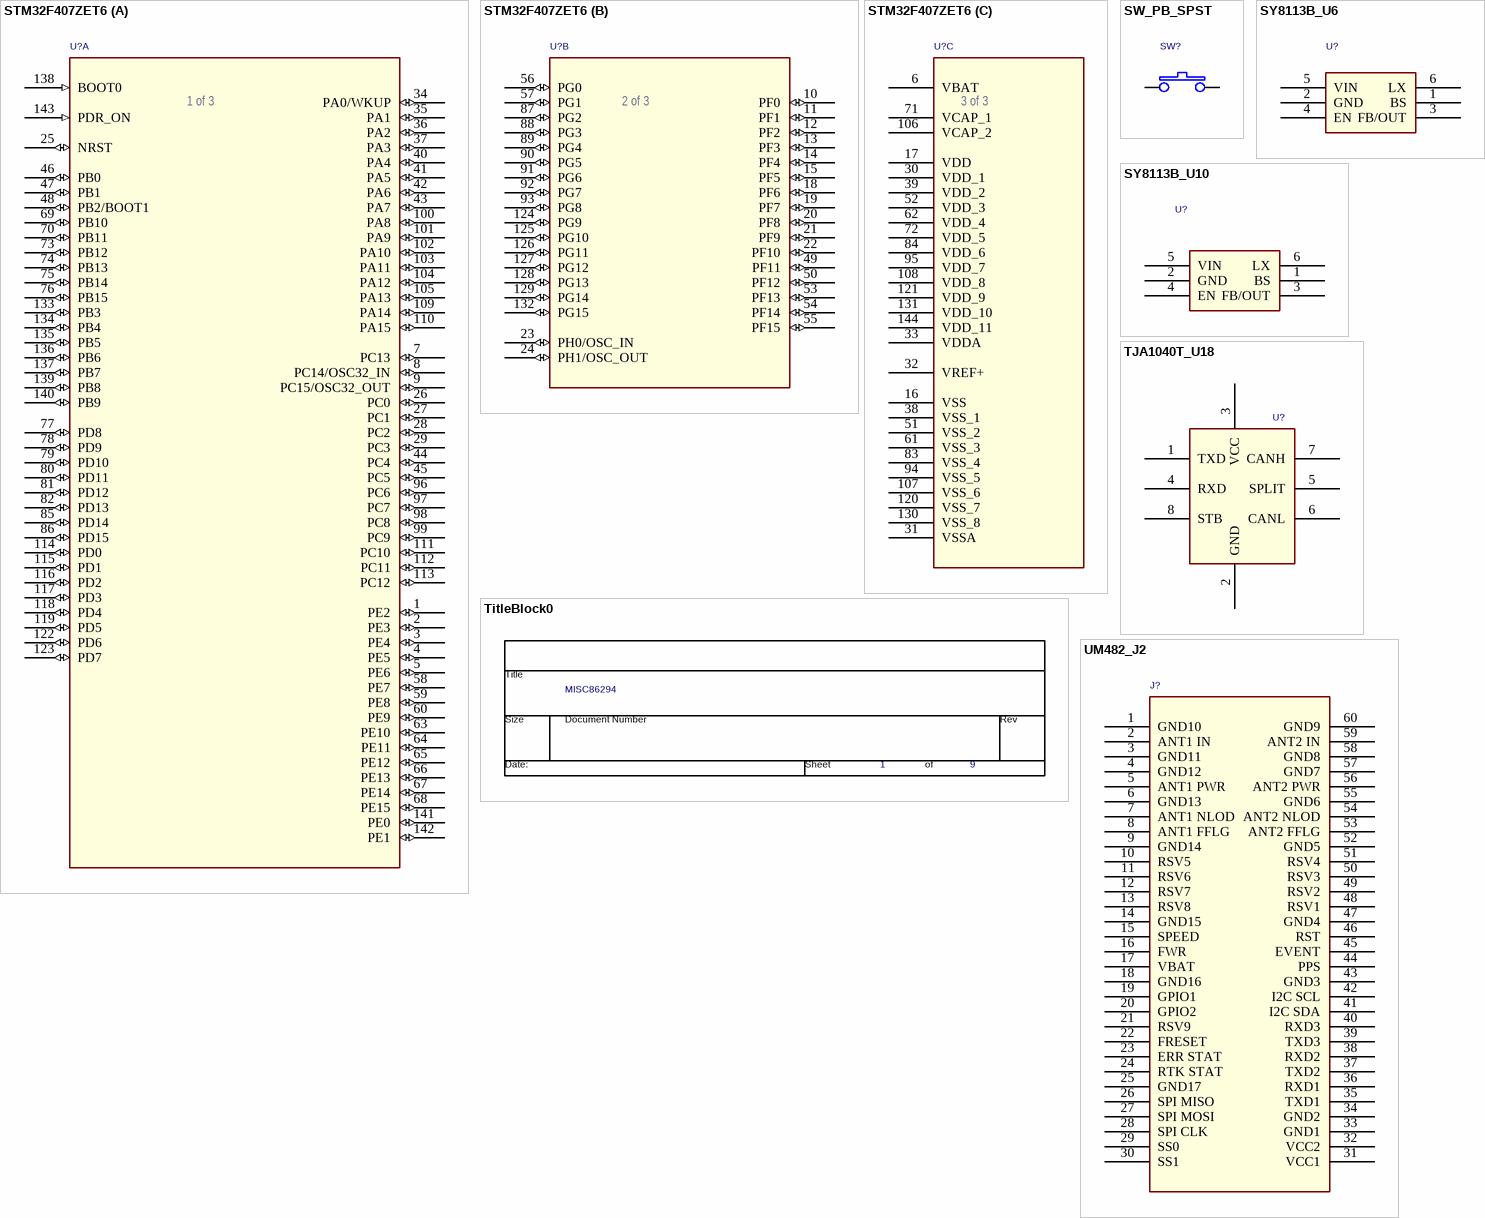
[diagram p6: symbols STM32F407ZET6 to UM482_J2]
## STM32F407ZET6
designator U?
footprint LQFP144-20x20mm
part A pins: 1 PE2 (io), 2 PE3 (io), 3 PE4 (io), 4 PE5 (io), 5 PE6 (io), 7 PC13 (io), 8 PC14/OSC32_IN (io), 9 PC15/OSC32_OUT (io), 25 NRST (io), 26 PC0 (io), 27 PC1 (io), 28 PC2 (io), 29 PC3 (io), 34 PA0/WKUP (io), 35 PA1 (io), 36 PA2 (io), 37 PA3 (io), 40 PA4 (io), 41 PA5 (io), 42 PA6 (io), 43 PA7 (io), 44 PC4 (io), 45 PC5 (io), 46 PB0 (io), 47 PB1 (io), 48 PB2/BOOT1 (io), 58 PE7 (io), 59 PE8 (io), 60 PE9 (io), 63 PE10 (io), 64 PE11 (io), 65 PE12 (io), 66 PE13 (io), 67 PE14 (io), 68 PE15 (io), 69 PB10 (io), 70 PB11 (io), 73 PB12 (io), 74 PB13 (io), 75 PB14 (io), 76 PB15 (io), 77 PD8 (io), 78 PD9 (io), 79 PD10 (io), 80 PD11 (io), 81 PD12 (io), 82 PD13 (io), 85 PD14 (io), 86 PD15 (io), 96 PC6 (io), 97 PC7 (io), 98 PC8 (io), 99 PC9 (io), 100 PA8 (io), 101 PA9 (io), 102 PA10 (io), 103 PA11 (io), 104 PA12 (io), 105 PA13 (io), 109 PA14 (io), 110 PA15 (io), 111 PC10 (io), 112 PC11 (io), 113 PC12 (io), 114 PD0 (io), 115 PD1 (io), 116 PD2 (io), 117 PD3 (io), 118 PD4 (io), 119 PD5 (io), 122 PD6 (io), 123 PD7 (io), 133 PB3 (io), 134 PB4 (io), 135 PB5 (io), 136 PB6 (io), 137 PB7 (io), 138 BOOT0 (in), 139 PB8 (io), 140 PB9 (io), 141 PE0 (io), 142 PE1 (io), 143 PDR_ON (in)
part B pins: 10 PF0 (io), 11 PF1 (io), 12 PF2 (io), 13 PF3 (io), 14 PF4 (io), 15 PF5 (io), 18 PF6 (io), 19 PF7 (io), 20 PF8 (io), 21 PF9 (io), 22 PF10 (io), 23 PH0/OSC_IN (io), 24 PH1/OSC_OUT (io), 49 PF11 (io), 50 PF12 (io), 53 PF13 (io), 54 PF14 (io), 55 PF15 (io), 56 PG0 (io), 57 PG1 (io), 87 PG2 (io), 88 PG3 (io), 89 PG4 (io), 90 PG5 (io), 91 PG6 (io), 92 PG7 (io), 93 PG8 (io), 124 PG9 (io), 125 PG10 (io), 126 PG11 (io), 127 PG12 (io), 128 PG13 (io), 129 PG14 (io), 132 PG15 (io)
part C pins: 6 VBAT (power), 16 VSS (power), 17 VDD (power), 30 VDD_1 (power), 31 VSSA (power), 32 VREF+ (power), 33 VDDA (power), 38 VSS_1 (power), 39 VDD_2 (power), 51 VSS_2 (power), 52 VDD_3 (power), 61 VSS_3 (power), 62 VDD_4 (power), 71 VCAP_1 (power), 72 VDD_5 (power), 83 VSS_4 (power), 84 VDD_6 (power), 94 VSS_5 (power), 95 VDD_7 (power), 106 VCAP_2 (power), 107 VSS_6 (power), 108 VDD_8 (power), 120 VSS_7 (power), 121 VDD_9 (power), 130 VSS_8 (power), 131 VDD_10 (power), 144 VDD_11 (power)

## SW_PB_SPST
designator SW?
footprint SMD
pins: 1, 2

## SY8113B_U6
designator U?
footprint TSOT-23-6_L2_9-W1_6-P0_95-LS2_8-BR
pins: 1 BS, 2 GND, 3 FB/OUT, 4 EN, 5 VIN, 6 LX

## SY8113B_U10
designator U?
footprint TSOT-23-6_L2_9-W1_6-P0_95-LS2_8-BR
pins: 1 BS, 2 GND, 3 FB/OUT, 4 EN, 5 VIN, 6 LX

## TitleBlock0
designator *?  Title: MISC86294  Page Number: 1  Page Count: 9  (graphical)

## TJA1040T_U18
designator U?
footprint SOIC-8
pins: 1 TXD, 2 GND, 3 VCC, 4 RXD, 5 SPLIT, 6 CANL, 7 CANH, 8 STB

## UM482_J2
designator J?
footprint UM482_K823
pins: 1 GND10, 2 ANT1 IN, 3 GND11, 4 GND12, 5 ANT1 PWR, 6 GND13, 7 ANT1 NLOD, 8 ANT1 FFLG, 9 GND14, 10 RSV5, 11 RSV6, 12 RSV7, 13 RSV8, 14 GND15, 15 SPEED, 16 FWR, 17 VBAT, 18 GND16, 19 GPIO1, 20 GPIO2, 21 RSV9, 22 FRESET, 23 ERR STAT, 24 RTK STAT, 25 GND17, 26 SPI MISO, 27 SPI MOSI, 28 SPI CLK, 29 SS0, 30 SS1, 31 VCC1, 32 VCC2, 33 GND1, 34 GND2, 35 TXD1, 36 RXD1, 37 TXD2, 38 RXD2, 39 TXD3, 40 RXD3, 41 I2C SDA, 42 I2C SCL, 43 GND3, 44 PPS, 45 EVENT, 46 RST, 47 GND4, 48 RSV1, 49 RSV2, 50 RSV3, 51 RSV4, 52 GND5, 53 ANT2 FFLG, 54 ANT2 NLOD, 55 GND6, 56 ANT2 PWR, 57 GND7, 58 GND8, 59 ANT2 IN, 60 GND9